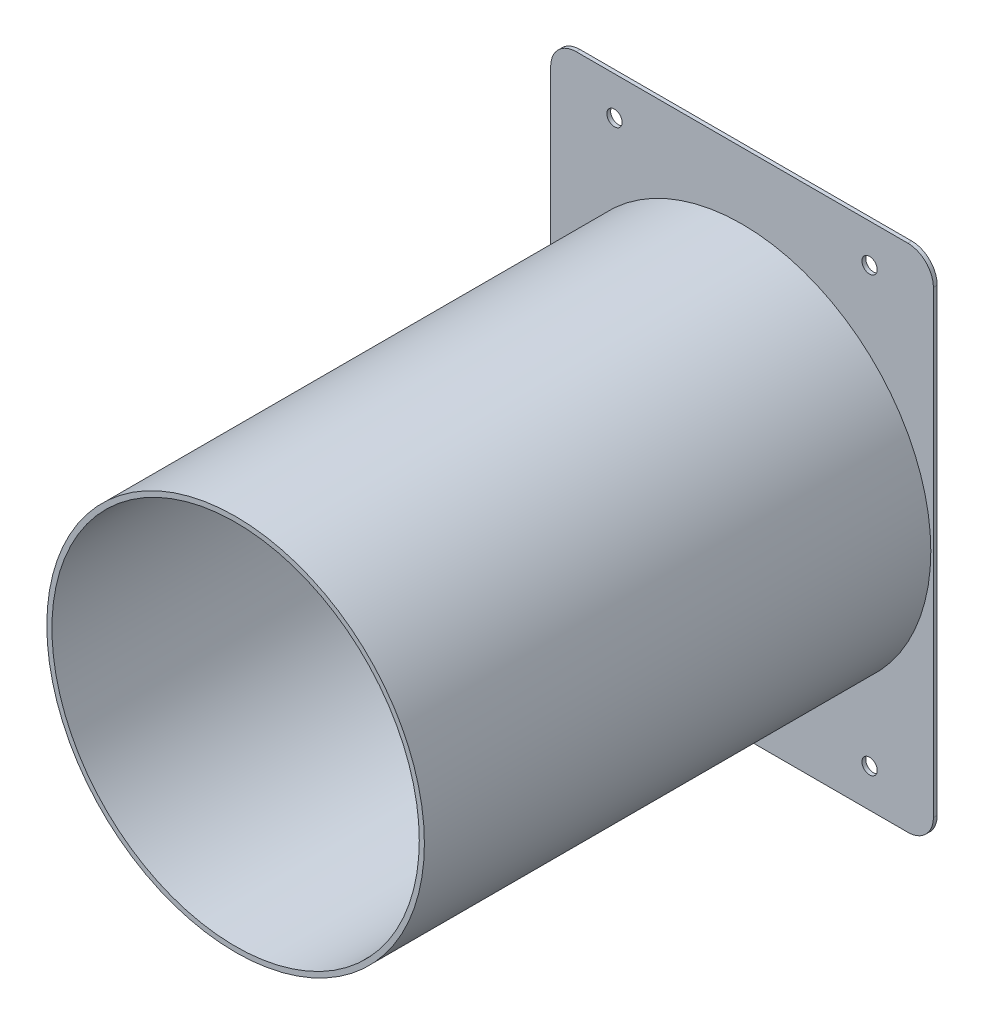
from build123d import *

# Parameters (mm, degrees)
SKETCH_1_R            = 74
SKETCH_1_R_2          = 72
EXTRUDE_1_DEPTH       = 200
SKETCH_2_W            = 150
SKETCH_2_H            = 200
SKETCH_2_R            = 74
EXTRUDE_2_DEPTH       = 1.5
FILLET_1_R            = 10
HOLE_WIZARD_6_0_6_1_D = 6


with BuildPart() as part:
    # 草图1 → 凸台-拉伸1 (new body)
    with BuildSketch(Plane.XY):
        Circle(SKETCH_1_R)
        Circle(SKETCH_1_R_2, mode=Mode.SUBTRACT)
    extrude(amount=EXTRUDE_1_DEPTH)

    # 草图2 → 凸台-拉伸2 (add)
    with BuildSketch(Plane(origin=(0, 0, 0), x_dir=(-1, 0, 0), z_dir=(0, 0, -1))):
        Rectangle(SKETCH_2_W, SKETCH_2_H)
        Circle(SKETCH_2_R, mode=Mode.SUBTRACT)
    extrude(amount=-EXTRUDE_2_DEPTH)

    # 圆角1
    fillet_1_edges = [part.edges().sort_by_distance(p)[0] for p in [
        (-75, 100, 0.75),
        (-75, -100, 0.75),
        (75, -100, 0.75),
        (75, 100, 0.75),
    ]]
    fillet(fillet_1_edges, radius=FILLET_1_R)

    # Ø6.0 (6) 直径孔1 (through all)
    with Locations(Plane.XY.offset(1.5)):
        with Locations((-50, -85), (-50, 85), (50, 85), (50, -85)):
            Hole(HOLE_WIZARD_6_0_6_1_D / 2)


solid = part.part
